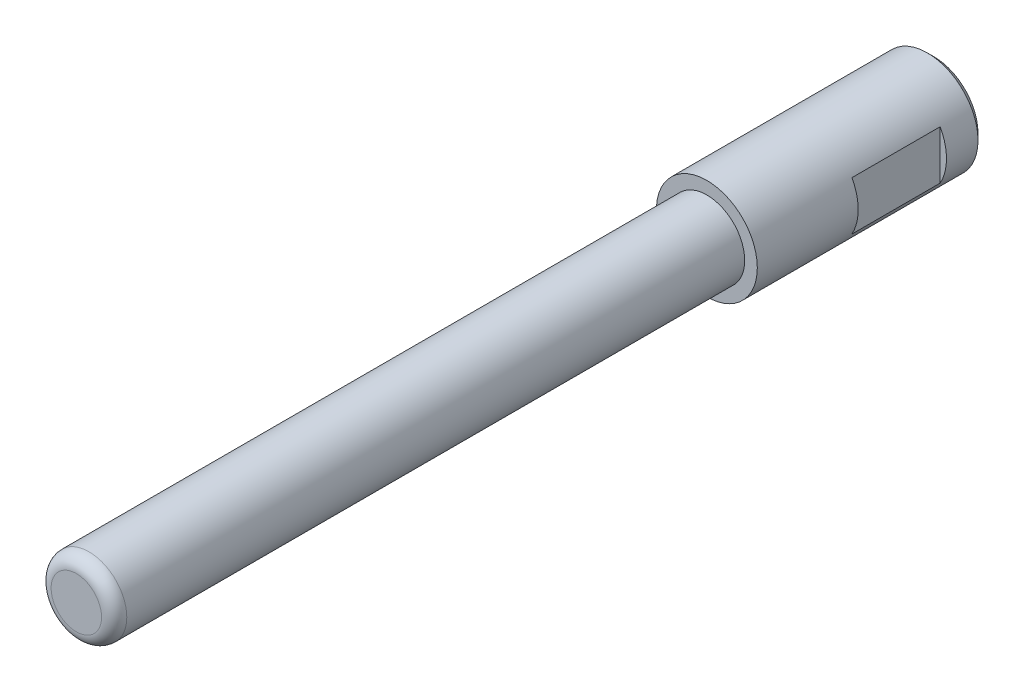
from build123d import *

# Parameters (mm, degrees)
SKETCH_1_R             = 4
EXTRUDE_1_DEPTH        = 18
SKETCH_2_R             = 3
EXTRUDE_2_DEPTH        = 50
FILLET_1_R             = 1
CHAMFER_1_SIZE         = 0.5
HOLE_WIZARD_M4_1_D     = 3.3
HOLE_WIZARD_M4_1_DEPTH = 13.5
HOLE_WIZARD_M4_1_TIP   = 0.991420021
SKETCH_5_W             = 2.600851977
SKETCH_5_H             = 9.759387418
SKETCH_5_W_2           = 4.309983276
SKETCH_5_H_2           = 9.585997286
CUT_EXTRUDE_1_DEPTH    = 7


with BuildPart() as part:
    # 草图1 → 凸台-拉伸1 (new body)
    with BuildSketch(Plane.XY):
        Circle(SKETCH_1_R)
    extrude(amount=EXTRUDE_1_DEPTH)

    # 草图2 → 凸台-拉伸2 (add)
    with BuildSketch(Plane.XY.offset(18)):
        Circle(SKETCH_2_R)
    extrude(amount=EXTRUDE_2_DEPTH)

    # 圆角1
    fillet_1_edges = [part.edges().sort_by_distance(p)[0] for p in [
        (-3, 0, 68),
    ]]
    fillet(fillet_1_edges, radius=FILLET_1_R)

    # 倒角1
    chamfer_1_edges = [part.edges().sort_by_distance(p)[0] for p in [
        (-4, 0, 0),
    ]]
    chamfer(chamfer_1_edges, length=CHAMFER_1_SIZE)

    # M4 螺纹孔1
    with Locations(Plane(origin=(0, 0, 0), x_dir=(-1, 0, 0), z_dir=(0, 0, -1))):
        with Locations((0, 0)):
            Hole(HOLE_WIZARD_M4_1_D / 2, depth=HOLE_WIZARD_M4_1_DEPTH)
            with Locations((0, 0, -(HOLE_WIZARD_M4_1_DEPTH + HOLE_WIZARD_M4_1_TIP / 2))):  # 118° drill point
                Cone(0, HOLE_WIZARD_M4_1_D / 2, HOLE_WIZARD_M4_1_TIP, mode=Mode.SUBTRACT)

    # 草图5 → 切除-拉伸1 (cut)
    with BuildSketch(Plane(origin=(0, 0, 3), x_dir=(-1, 0, 0), z_dir=(0, 0, -1))):
        with Locations((-4.800425989, -0.334395254)):
            Rectangle(SKETCH_5_W, SKETCH_5_H)
        with Locations((5.654991638, -0.247700188)):
            Rectangle(SKETCH_5_W_2, SKETCH_5_H_2)
    extrude(amount=-CUT_EXTRUDE_1_DEPTH, mode=Mode.SUBTRACT)


solid = part.part
